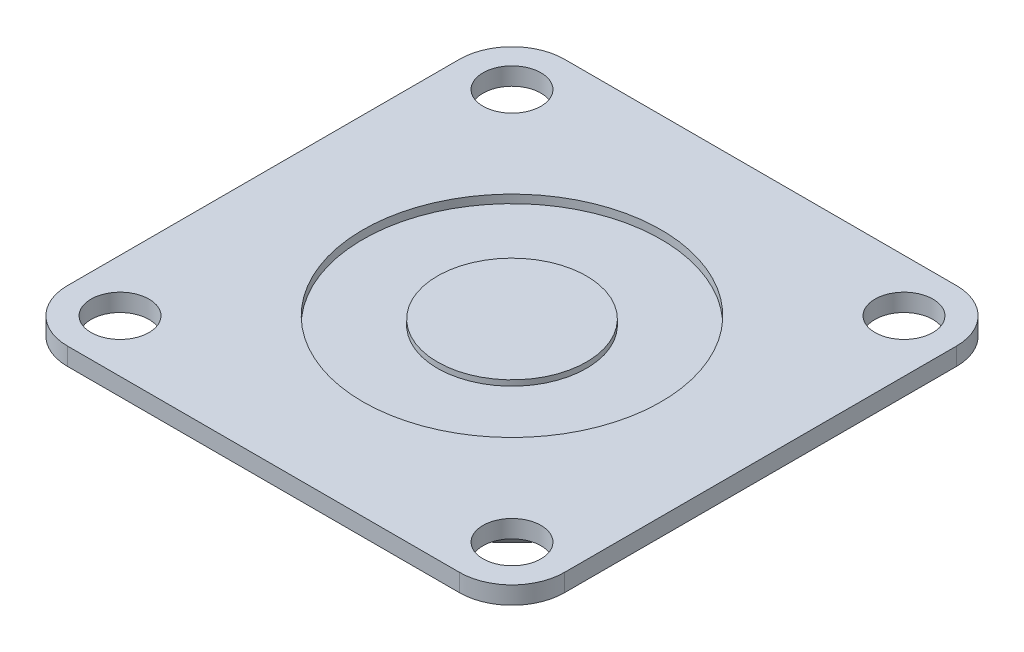
from build123d import *

# Parameters (mm, degrees)
SKETCH_1_R          = 5.25
EXTRUDE_1_DEPTH     = 3.2
SKETCH_2_R          = 27
CUT_EXTRUDE_1_DEPTH = 1.5
SKETCH_3_R          = 13.5
EXTRUDE_2_DEPTH     = 1


with BuildPart() as part:
    # 草图1 → 凸台-拉伸1 (new body)
    with BuildSketch(Plane(origin=(0, 0, 0), x_dir=(1, 0, 0), z_dir=(0, 1, 0))):
        with BuildLine():
            Line((-35.5, -45), (35.5, -45))
            ThreePointArc((35.5, -45), (42.217514421, -42.217514421), (45, -35.5))
            Line((45, -35.5), (45, 35.5))
            ThreePointArc((45, 35.5), (42.217514421, 42.217514421), (35.5, 45))
            Line((35.5, 45), (-35.5, 45))
            ThreePointArc((-35.5, 45), (-42.217514421, 42.217514421), (-45, 35.5))
            Line((-45, 35.5), (-45, -35.5))
            ThreePointArc((-45, -35.5), (-42.217514421, -42.217514421), (-35.5, -45))
        make_face()
        with Locations(Location((35.5, -35.5, 0), (0, 0, 270))):
            Circle(SKETCH_1_R, mode=Mode.SUBTRACT)
        with Locations(Location((35.5, 35.5, 0), (0, 0, 270))):
            Circle(SKETCH_1_R, mode=Mode.SUBTRACT)
        with Locations(Location((-35.5, -35.5, 0), (0, 0, 270))):
            Circle(SKETCH_1_R, mode=Mode.SUBTRACT)
        with Locations(Location((-35.5, 35.5, 0), (0, 0, 270))):
            Circle(SKETCH_1_R, mode=Mode.SUBTRACT)
    extrude(amount=-EXTRUDE_1_DEPTH)

    # 草图2 → 切除-拉伸1 (cut)
    with BuildSketch(Plane(origin=(0, 0, 0), x_dir=(1, 0, 0), z_dir=(0, 1, 0))):
        with Locations(Location((0, 0, 0), (0, 0, 270))):
            Circle(SKETCH_2_R)
    extrude(amount=-CUT_EXTRUDE_1_DEPTH, mode=Mode.SUBTRACT)

    # 草图3 → 凸台-拉伸2 (add)
    with BuildSketch(Plane(origin=(0, -1.5, 0), x_dir=(1, 0, 0), z_dir=(0, 1, 0))):
        with Locations(Location((0, 0, 0), (0, 0, 270))):
            Circle(SKETCH_3_R)
    extrude(amount=EXTRUDE_2_DEPTH)

    # 草图4 → 旋转1 (revolve)
    with BuildSketch(Plane(origin=(0, 0, 0), x_dir=(0, 0, -1), z_dir=(1, 0, 0))):
        with BuildLine():
            Line((0, -14.2), (-29.255663301, -14.2))
            ThreePointArc((-29.255663301, -14.2), (-31.091107897, -13.621286542), (-32.262679687, -12.094464459))
            Line((-32.262679687, -12.094464459), (-35.5, -3.2))
            Line((-35.5, -3.2), (0, -3.2))
            Line((0, -3.2), (0, -14.2))
        make_face()
    revolve(axis=Axis((0, -3.2, 0), (0, -1, 0)))


solid = part.part
